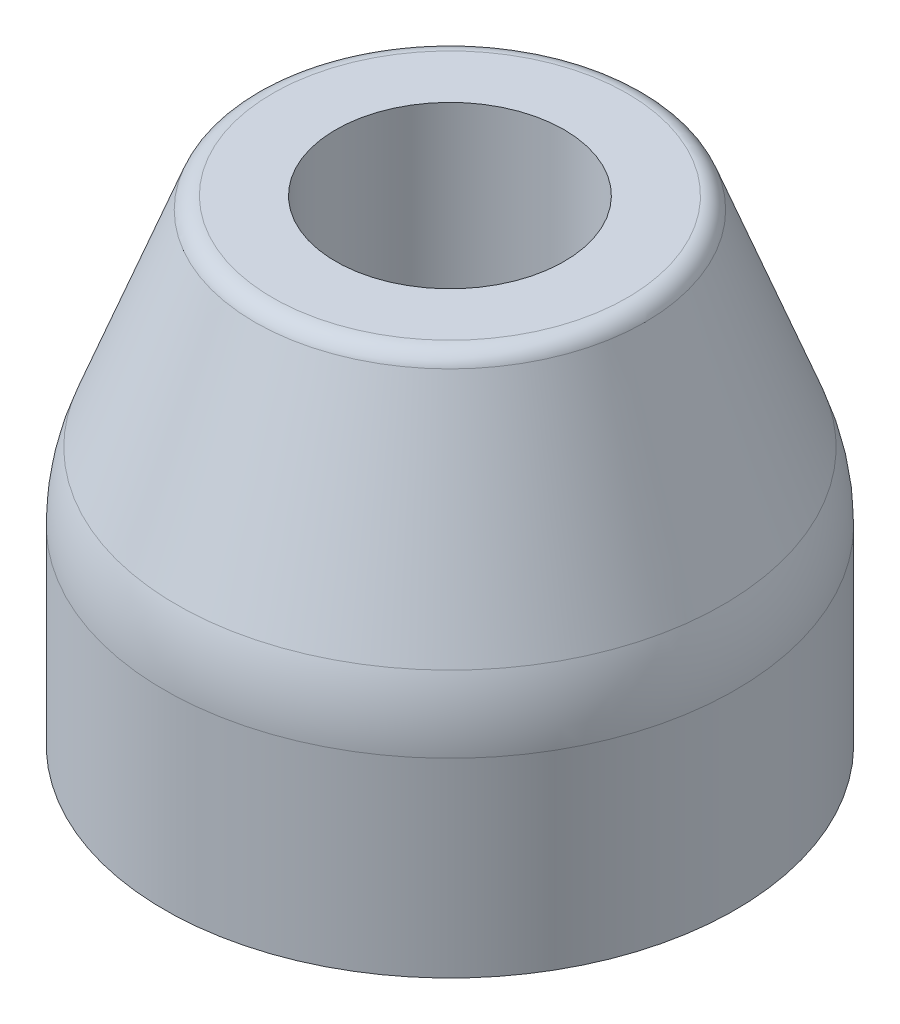
from build123d import *


with BuildPart() as part:
    # Sketch1 → Revolve1 (revolve)
    with BuildSketch(Plane.XY, mode=Mode.PRIVATE) as revolve1_sk:
        with BuildLine():
            Line((4, 0), (4, 11))
            Line((4, 11), (6, 11))
            Line((6, 11), (6, 25))
            Line((6, 25), (9.310102051, 25))
            ThreePointArc((9.310102051, 25), (9.877970423, 24.823119379), (10.244948974, 24.355051026))
            Line((10.244948974, 24.355051026), (14.348469228, 13.550510257))
            ThreePointArc((14.348469228, 13.550510257), (14.835768711, 11.804897188), (15, 10))
            Line((15, 10), (15, 0))
            Line((15, 0), (4, 0))
        make_face()
    revolve(revolve1_sk.sketch.rotate(Axis((0, 0, 0), (0, 1, 0)), 90), axis=Axis((0, 0, 0), (0, 1, 0)))


solid = part.part
